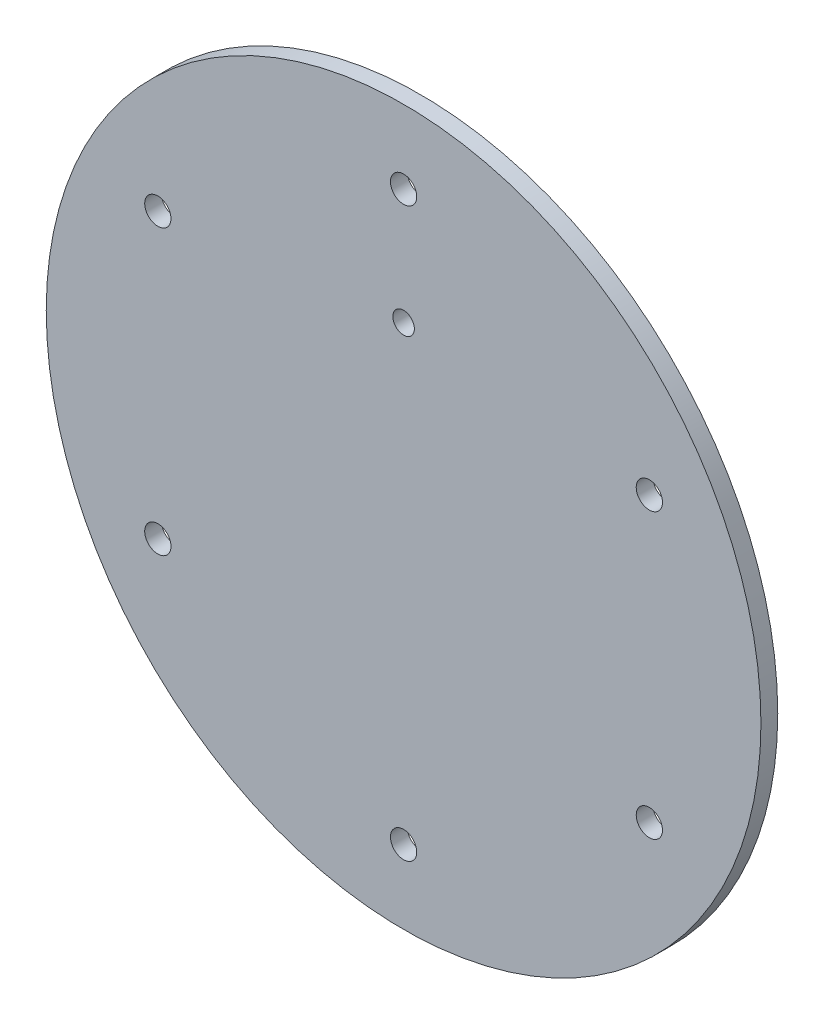
from build123d import *

# Parameters (mm, degrees)
SKETCH1_R           = 170
BOSS_EXTRUDE1_DEPTH = 8
SKETCH3_R           = 6.25
CUT_EXTRUDE1_DEPTH  = 10
SKETCH4_R           = 5.125
CUT_EXTRUDE2_DEPTH  = 10


with BuildPart() as part:
    # Sketch1 → Boss-Extrude1 (new body)
    with BuildSketch(Plane.XY):
        Circle(SKETCH1_R)
    extrude(amount=BOSS_EXTRUDE1_DEPTH)

    # Sketch3 → Cut-Extrude1 (cut)
    with BuildSketch(Plane(origin=(0, 0, 0), x_dir=(-1, 0, 0), z_dir=(0, 0, -1))):
        with Locations((116.913429511, 67.5)):
            Circle(SKETCH3_R)
        with Locations((0, 135)):
            Circle(SKETCH3_R)
        with Locations((116.913429511, -67.5)):
            Circle(SKETCH3_R)
        with Locations((0, -135)):
            Circle(SKETCH3_R)
        with Locations((-116.913429511, -67.5)):
            Circle(SKETCH3_R)
        with Locations((-116.913429511, 67.5)):
            Circle(SKETCH3_R)
    extrude(amount=-CUT_EXTRUDE1_DEPTH, mode=Mode.SUBTRACT)

    # Sketch4 → Cut-Extrude2 (cut)
    with BuildSketch(Plane(origin=(0, 0, 0), x_dir=(-1, 0, 0), z_dir=(0, 0, -1))):
        with Locations((0, 80)):
            Circle(SKETCH4_R)
    extrude(amount=-CUT_EXTRUDE2_DEPTH, mode=Mode.SUBTRACT)


solid = part.part
